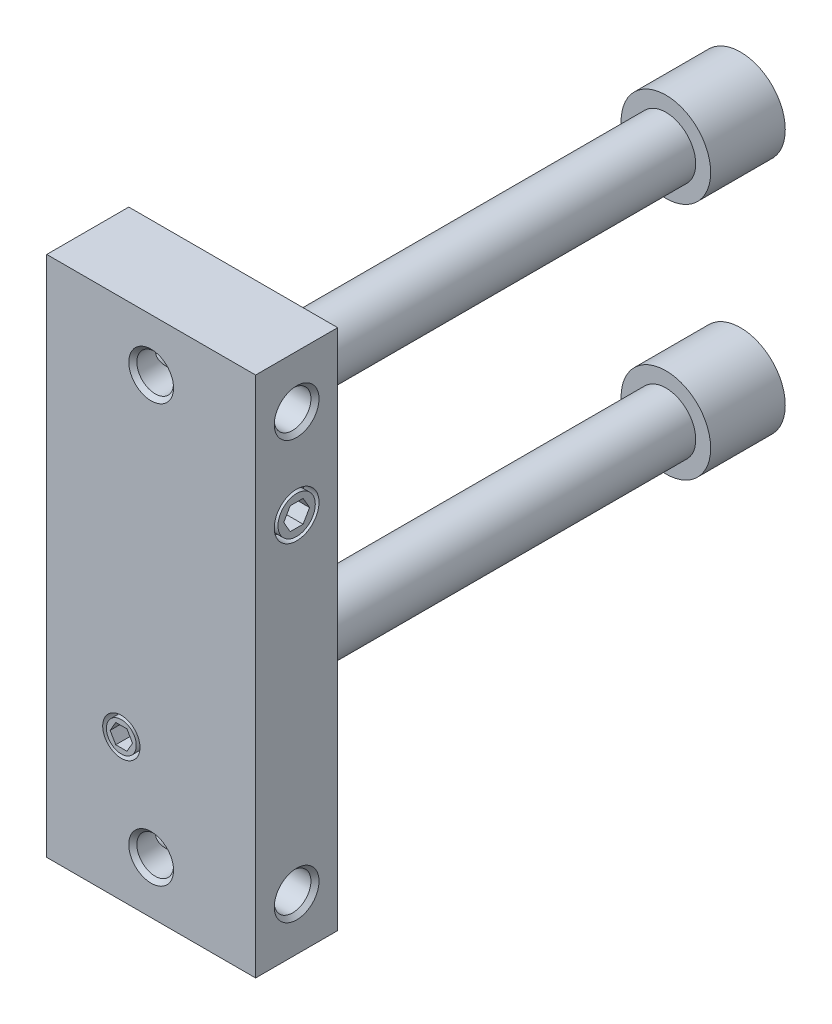
from build123d import *

# Parameters (mm, degrees)
SKETCH1_W           = 14
SKETCH1_H           = 35
BOSS_EXTRUDE1_DEPTH = 5.5
SKETCH8_R           = 1.25
SKETCH8_R_2         = 1
CUT_EXTRUDE1_DEPTH  = 1
CUT_EXTRUDE2_DEPTH  = 1.3
SKETCH10_R          = 1.5
SKETCH10_R_2        = 1.25
CUT_EXTRUDE3_DEPTH  = 1
CUT_EXTRUDE4_DEPTH  = 1.5


with BuildPart() as part:
    # Sketch1 → Boss-Extrude1 (new body)
    with BuildSketch(Plane.XY.offset(8)):
        with Locations((2, 0)):
            Rectangle(SKETCH1_W, SKETCH1_H)
    extrude(amount=BOSS_EXTRUDE1_DEPTH)

    # Sketch2 → Revolve1 (revolve)
    with BuildSketch(Plane(origin=(0, 0, 0), x_dir=(0, 0, -1), z_dir=(1, 0, 0)), mode=Mode.PRIVATE) as revolve1_sk:
        Polygon((-13, 8), (-13, 10), (23, 10), (23, 11), (28, 11), (28, 8), align=None)
    revolve(revolve1_sk.sketch.rotate(Axis((0, 8, -28), (0, 0, 1)), 270), axis=Axis((0, 8, -28), (0, 0, 1)))

    # Sketch3 → Revolve2 (revolve)
    with BuildSketch(Plane(origin=(0, 0, 0), x_dir=(0, 0, -1), z_dir=(1, 0, 0)), mode=Mode.PRIVATE) as revolve2_sk:
        Polygon((-13, -8), (-13, -6), (23, -6), (23, -5), (28, -5), (28, -8), align=None)
    revolve(revolve2_sk.sketch.rotate(Axis((0, -8, -28), (0, 0, 1)), 270), axis=Axis((0, -8, -28), (0, 0, 1)))

    # Sketch4 → Cut-Revolve1 (revolve, cut)
    with BuildSketch(Plane(origin=(2, 0, 0), x_dir=(0, 0, -1), z_dir=(1, 0, 0)), mode=Mode.PRIVATE) as cut_revolve1_sk:
        Polygon((-13.5, 14), (-13.5, 15.5), (-13.2295, 15.2295), (-8.2705, 15.2295), (-8, 15.5), (-8, 14), align=None)
    revolve(cut_revolve1_sk.sketch.rotate(Axis((2, 14, 8), (0, 0, 1)), 270), axis=Axis((2, 14, 8), (0, 0, 1)), mode=Mode.SUBTRACT)

    # Sketch5 → Cut-Revolve2 (revolve, cut)
    with BuildSketch(Plane(origin=(2, 0, 0), x_dir=(0, 0, -1), z_dir=(1, 0, 0)), mode=Mode.PRIVATE) as cut_revolve2_sk:
        Polygon((-13.5, -14), (-13.5, -12.5), (-13.2295, -12.7705), (-8.2705, -12.7705), (-8, -12.5), (-8, -14), align=None)
    revolve(cut_revolve2_sk.sketch.rotate(Axis((2, -14, 8), (0, 0, 1)), 270), axis=Axis((2, -14, 8), (0, 0, 1)), mode=Mode.SUBTRACT)

    # Sketch6 → Cut-Revolve3 (revolve, cut)
    with BuildSketch(Plane.XY.offset(10.75), mode=Mode.PRIVATE) as cut_revolve3_sk:
        Polygon((-5, 14), (-5, 15.5), (-4.7295, 15.2295), (8.7295, 15.2295), (9, 15.5), (9, 14), align=None)
    revolve(cut_revolve3_sk.sketch.rotate(Axis((9, 14, 10.75), (-1, 0, 0)), 270), axis=Axis((9, 14, 10.75), (-1, 0, 0)), mode=Mode.SUBTRACT)

    # Sketch7 → Cut-Revolve4 (revolve, cut)
    with BuildSketch(Plane.XY.offset(10.75), mode=Mode.PRIVATE) as cut_revolve4_sk:
        Polygon((-5, -14), (-5, -12.5), (-4.7295, -12.7705), (8.7295, -12.7705), (9, -12.5), (9, -14), align=None)
    revolve(cut_revolve4_sk.sketch.rotate(Axis((9, -14, 10.75), (-1, 0, 0)), 270), axis=Axis((9, -14, 10.75), (-1, 0, 0)), mode=Mode.SUBTRACT)

    # Sketch8 → Cut-Extrude1 (cut)
    with BuildSketch(Plane.XY.offset(13.5)):
        with Locations((0, -8)):
            Circle(SKETCH8_R)
        with Locations((0, -8)):
            Circle(SKETCH8_R_2, mode=Mode.SUBTRACT)
    extrude(amount=-CUT_EXTRUDE1_DEPTH, mode=Mode.SUBTRACT)

    # Sketch9 → Cut-Extrude2 (cut)
    with BuildSketch(Plane.XY.offset(13.5)):
        Polygon((-0.75055535, -8), (-0.375277675, -8.65), (0.375277675, -8.65), (0.75055535, -8), (0.375277675, -7.35), (-0.375277675, -7.35), align=None)
    extrude(amount=-CUT_EXTRUDE2_DEPTH, mode=Mode.SUBTRACT)

    # Sketch10 → Cut-Extrude3 (cut)
    with BuildSketch(Plane(origin=(9, 0, 0), x_dir=(0, 0, -1), z_dir=(1, 0, 0))):
        with Locations((-10.75, 8)):
            Circle(SKETCH10_R)
        with Locations((-10.75, 8)):
            Circle(SKETCH10_R_2, mode=Mode.SUBTRACT)
    extrude(amount=-CUT_EXTRUDE3_DEPTH, mode=Mode.SUBTRACT)

    # Sketch11 → Cut-Extrude4 (cut)
    with BuildSketch(Plane(origin=(9, 0, 0), x_dir=(0, 0, -1), z_dir=(1, 0, 0))):
        Polygon((-11.616025404, 8), (-11.183012702, 7.25), (-10.316987298, 7.25), (-9.883974596, 8), (-10.316987298, 8.75), (-11.183012702, 8.75), align=None)
    extrude(amount=-CUT_EXTRUDE4_DEPTH, mode=Mode.SUBTRACT)


solid = part.part
